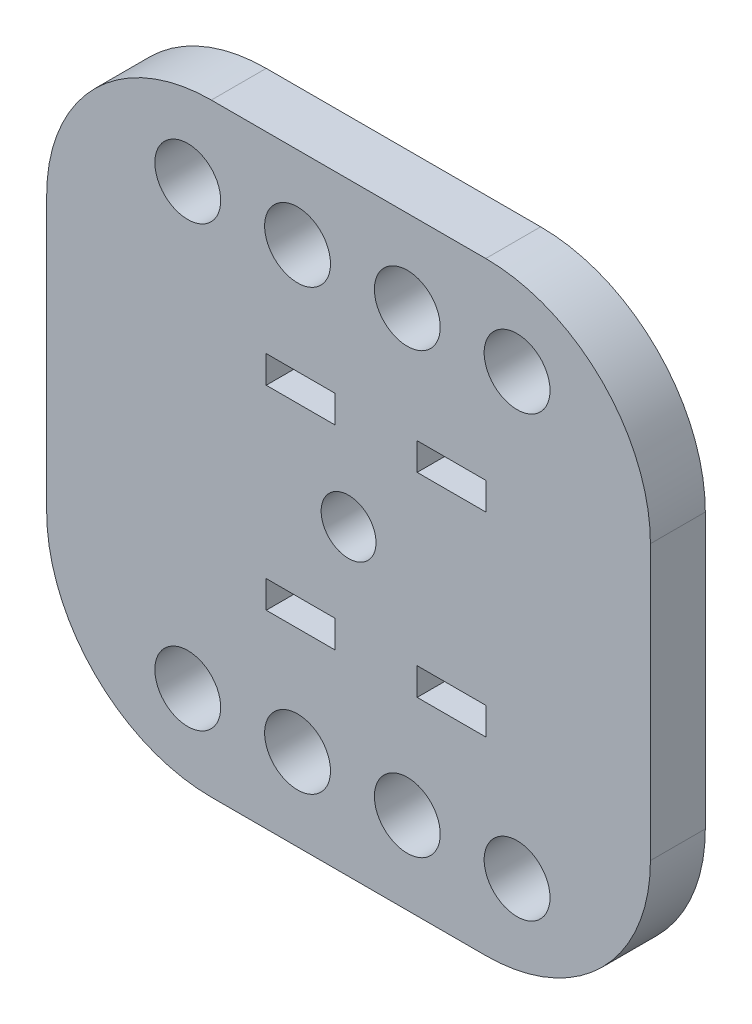
from build123d import *

# Parameters (mm, degrees)
SKETCH_1_R          = 6
SKETCH_1_W          = 12.5
SKETCH_1_H          = 5
EXTRUDE_1_DEPTH     = 10
SKETCH_2_R          = 11
EXTRUDE_2_DEPTH     = 15
SKETCH_3_R          = 5
CUT_EXTRUDE_1_DEPTH = 25
FILLET_1_R          = 0.5
FILLET_2_R          = 0.5


with BuildPart() as part:
    # 草图1 → 凸台-拉伸1 (new body)
    with BuildSketch(Plane.XY):
        with BuildLine():
            Line((-25.422431237, 54.841573229), (24.577568763, 54.841573229))
            ThreePointArc((24.577568763, 54.841573229), (45.790772199, 46.054776665), (54.577568763, 24.841573229))
            Line((54.577568763, 24.841573229), (54.577568763, -25.158426771))
            ThreePointArc((54.577568763, -25.158426771), (45.790772199, -46.371630206), (24.577568763, -55.158426771))
            Line((24.577568763, -55.158426771), (-25.422431237, -55.158426771))
            ThreePointArc((-25.422431237, -55.158426771), (-46.635634673, -46.371630206), (-55.422431237, -25.158426771))
            Line((-55.422431237, -25.158426771), (-55.422431237, 24.841573229))
            ThreePointArc((-55.422431237, 24.841573229), (-46.635634673, 46.054776665), (-25.422431237, 54.841573229))
        make_face()
        with Locations((-29.718021333, 39.841573229)):
            Circle(SKETCH_1_R, mode=Mode.SUBTRACT)
        with Locations((-9.718021333, 39.841573229)):
            Circle(SKETCH_1_R, mode=Mode.SUBTRACT)
        with Locations((10.281978667, 39.841573229)):
            Circle(SKETCH_1_R, mode=Mode.SUBTRACT)
        with Locations((30.281978667, 39.841573229)):
            Circle(SKETCH_1_R, mode=Mode.SUBTRACT)
        with Locations((30.281978667, -40.158426771)):
            Circle(SKETCH_1_R, mode=Mode.SUBTRACT)
        with Locations((10.281978667, -40.158426771)):
            Circle(SKETCH_1_R, mode=Mode.SUBTRACT)
        with Locations((-9.718021333, -40.158426771)):
            Circle(SKETCH_1_R, mode=Mode.SUBTRACT)
        with Locations((-29.718021333, -40.158426771)):
            Circle(SKETCH_1_R, mode=Mode.SUBTRACT)
        with Locations((18.327568763, 17.341573229)):
            Rectangle(SKETCH_1_W, SKETCH_1_H, mode=Mode.SUBTRACT)
        with Locations((18.327568763, -18.158426771)):
            Rectangle(SKETCH_1_W, SKETCH_1_H, mode=Mode.SUBTRACT)
        with Locations((-9.172431237, -18.158426771)):
            Rectangle(SKETCH_1_W, SKETCH_1_H, mode=Mode.SUBTRACT)
        with Locations((-9.172431237, 17.341573229)):
            Rectangle(SKETCH_1_W, SKETCH_1_H, mode=Mode.SUBTRACT)
    extrude(amount=EXTRUDE_1_DEPTH)

    # 草图2 → 凸台-拉伸2 (add)
    with BuildSketch(Plane(origin=(0, 0, 0), x_dir=(-1, 0, 0), z_dir=(0, 0, -1))):
        with Locations(Location((0.422431237, 0, 0), (0, 0, 180))):
            Circle(SKETCH_2_R)
    extrude(amount=EXTRUDE_2_DEPTH)

    # 草图3 → 切除-拉伸1 (cut)
    with BuildSketch(Plane(origin=(0, 0, -15), x_dir=(-1, 0, 0), z_dir=(0, 0, -1))):
        with Locations((0.422431237, 0)):
            Circle(SKETCH_3_R)
    extrude(amount=-CUT_EXTRUDE_1_DEPTH, mode=Mode.SUBTRACT)

    # 圆角1
    fillet_1_edges = [part.edges().sort_by_distance(p)[0] for p in [
        (4.577568763, 0, -15),
    ]]
    fillet(fillet_1_edges, radius=FILLET_1_R)

    # 圆角2
    fillet_2_edges = [part.edges().sort_by_distance(p)[0] for p in [
        (-11.422431237, 0, -15),
    ]]
    fillet(fillet_2_edges, radius=FILLET_2_R)


solid = part.part
